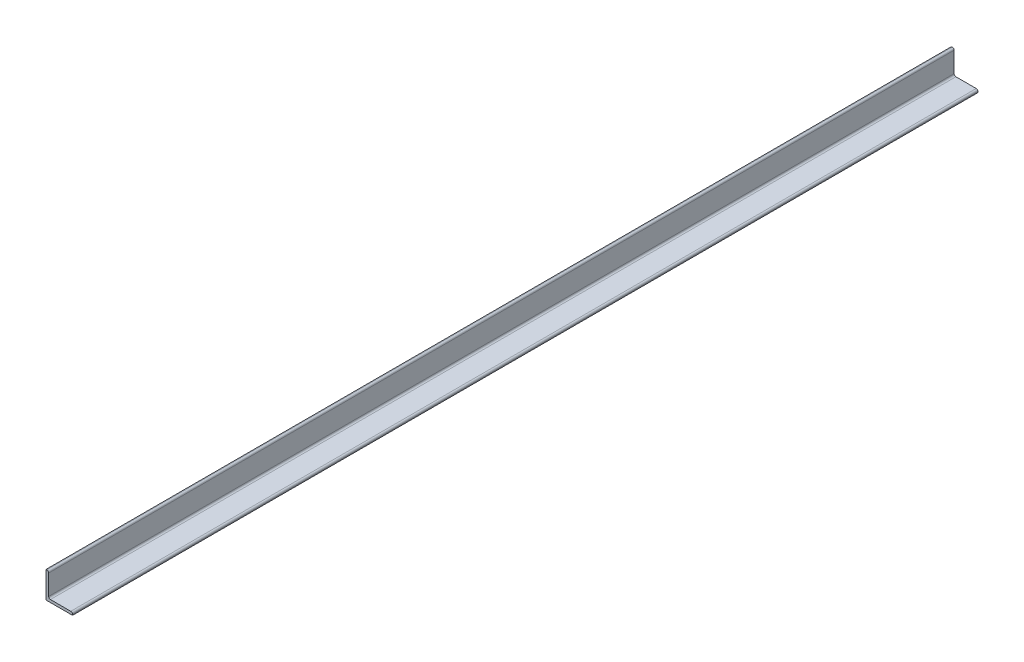
SolidWorks part; units mm, degrees
material "Plain Carbon Steel"
ref_plane "Front Plane" through (0, 0, 0) normal (0, 0, 1) x (1, 0, 0)
ref_plane "Top Plane" through (0, 0, 0) normal (0, 1, 0) x (1, 0, 0)
ref_plane "Right Plane" through (0, 0, 0) normal (1, 0, 0) x (0, 0, -1)
sketch "Sketch1" plane through (0, 0, 0) normal (0, 0, 1) x (1, 0, 0)
  line L0 (0, 0) -> (30, 0)
  line L1 (0, 0) -> (0, 30)
  line L2 (5, 3) -> (28, 3)
  line L3 (3, 5) -> (3, 28)
  line L4 (0, 30) -> (1, 30)
  line L5 (30, 1) -> (30, 0)
  line L6 (3, 3) -> (30, 3) construction
  line L7 (3, 3) -> (3, 30) construction
  arc A0 (30, 1) -> (28, 3) centre (28, 1) ccw
  arc A1 (5, 3) -> (3, 5) centre (5, 5) cw
  arc A2 (3, 28) -> (1, 30) centre (1, 28) ccw
  dimension "D4" = 2
  dimension "D1" = 30
  dimension "D2" = 30
  dimension "D3" = 3
extrude "Boss-Extrude1" add sketch "Sketch1" along normal blind 1024
